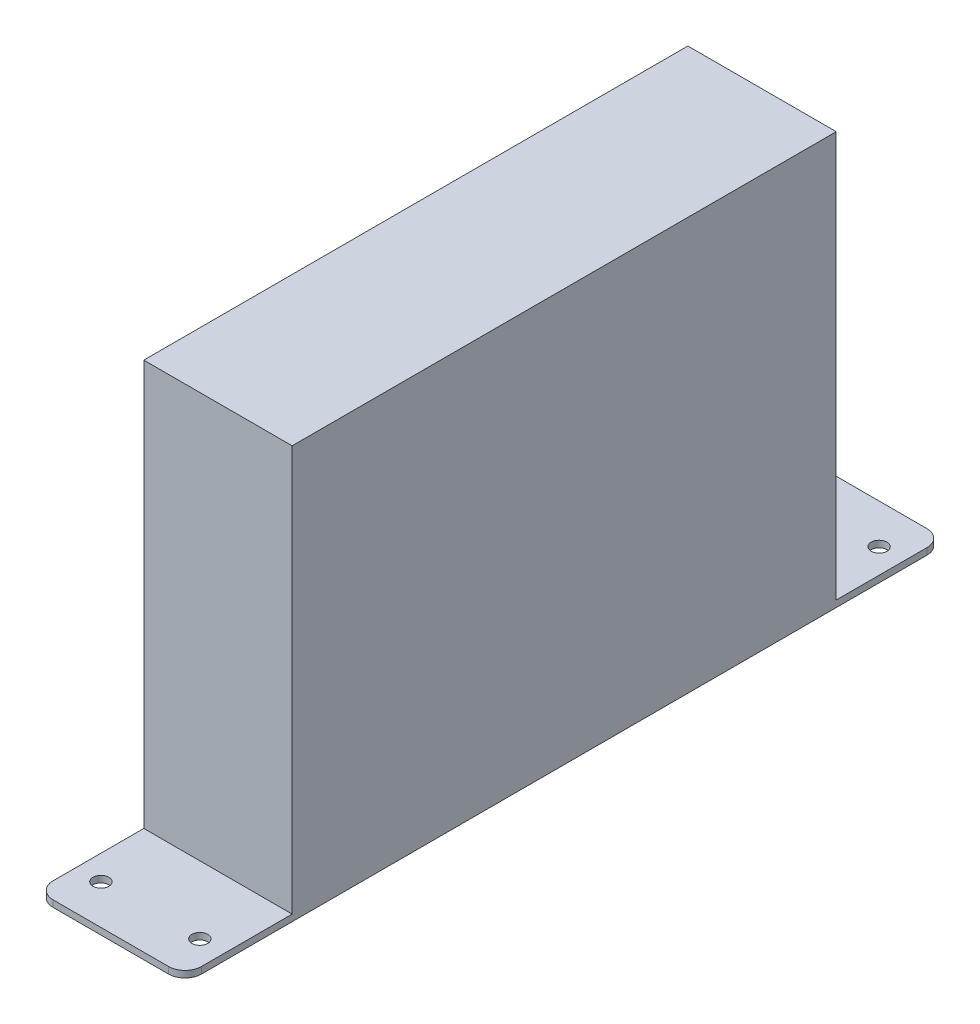
from build123d import *

# Parameters (mm, degrees)
SKETCH_1_W         = 45
SKETCH_1_H         = 165
EXTRUDE_1_DEPTH    = 125
SKETCH_3_W         = 45
SKETCH_3_H         = 32.5
EXTRUDE_2_DEPTH    = 2
HOLE_WIZARD_M4_1_D = 4.8
FILLET_1_R         = 5


with BuildPart() as part:
    # 草图1 → 凸台-拉伸1 (new body)
    with BuildSketch(Plane(origin=(0, 0, 0), x_dir=(1, 0, 0), z_dir=(0, 1, 0))):
        Rectangle(SKETCH_1_W, SKETCH_1_H)
    extrude(amount=EXTRUDE_1_DEPTH)

    # 草图3 → 凸台-拉伸2 (add)
    with BuildSketch(Plane(origin=(0, 0, 0), x_dir=(1, 0, 0), z_dir=(0, 1, 0))):
        with Locations((0, 98.75)):
            Rectangle(SKETCH_3_W, SKETCH_3_H)
        with Locations((0, -98.75)):
            Rectangle(SKETCH_3_W, SKETCH_3_H)
    extrude(amount=EXTRUDE_2_DEPTH)

    # M4 间隙孔1 (through all)
    with Locations(Plane(origin=(0, 2, 0), x_dir=(1, 0, 0), z_dir=(0, 1, 0))):
        with Locations((-15, 103), (15, 103), (15, -103), (-15, -103)):
            Hole(HOLE_WIZARD_M4_1_D / 2)

    # 圆角1
    fillet_1_edges = [part.edges().sort_by_distance(p)[0] for p in [
        (-22.5, 1, -115),
        (22.5, 1, -115),
        (-22.5, 1, 115),
        (22.5, 1, 115),
    ]]
    fillet(fillet_1_edges, radius=FILLET_1_R)


solid = part.part
